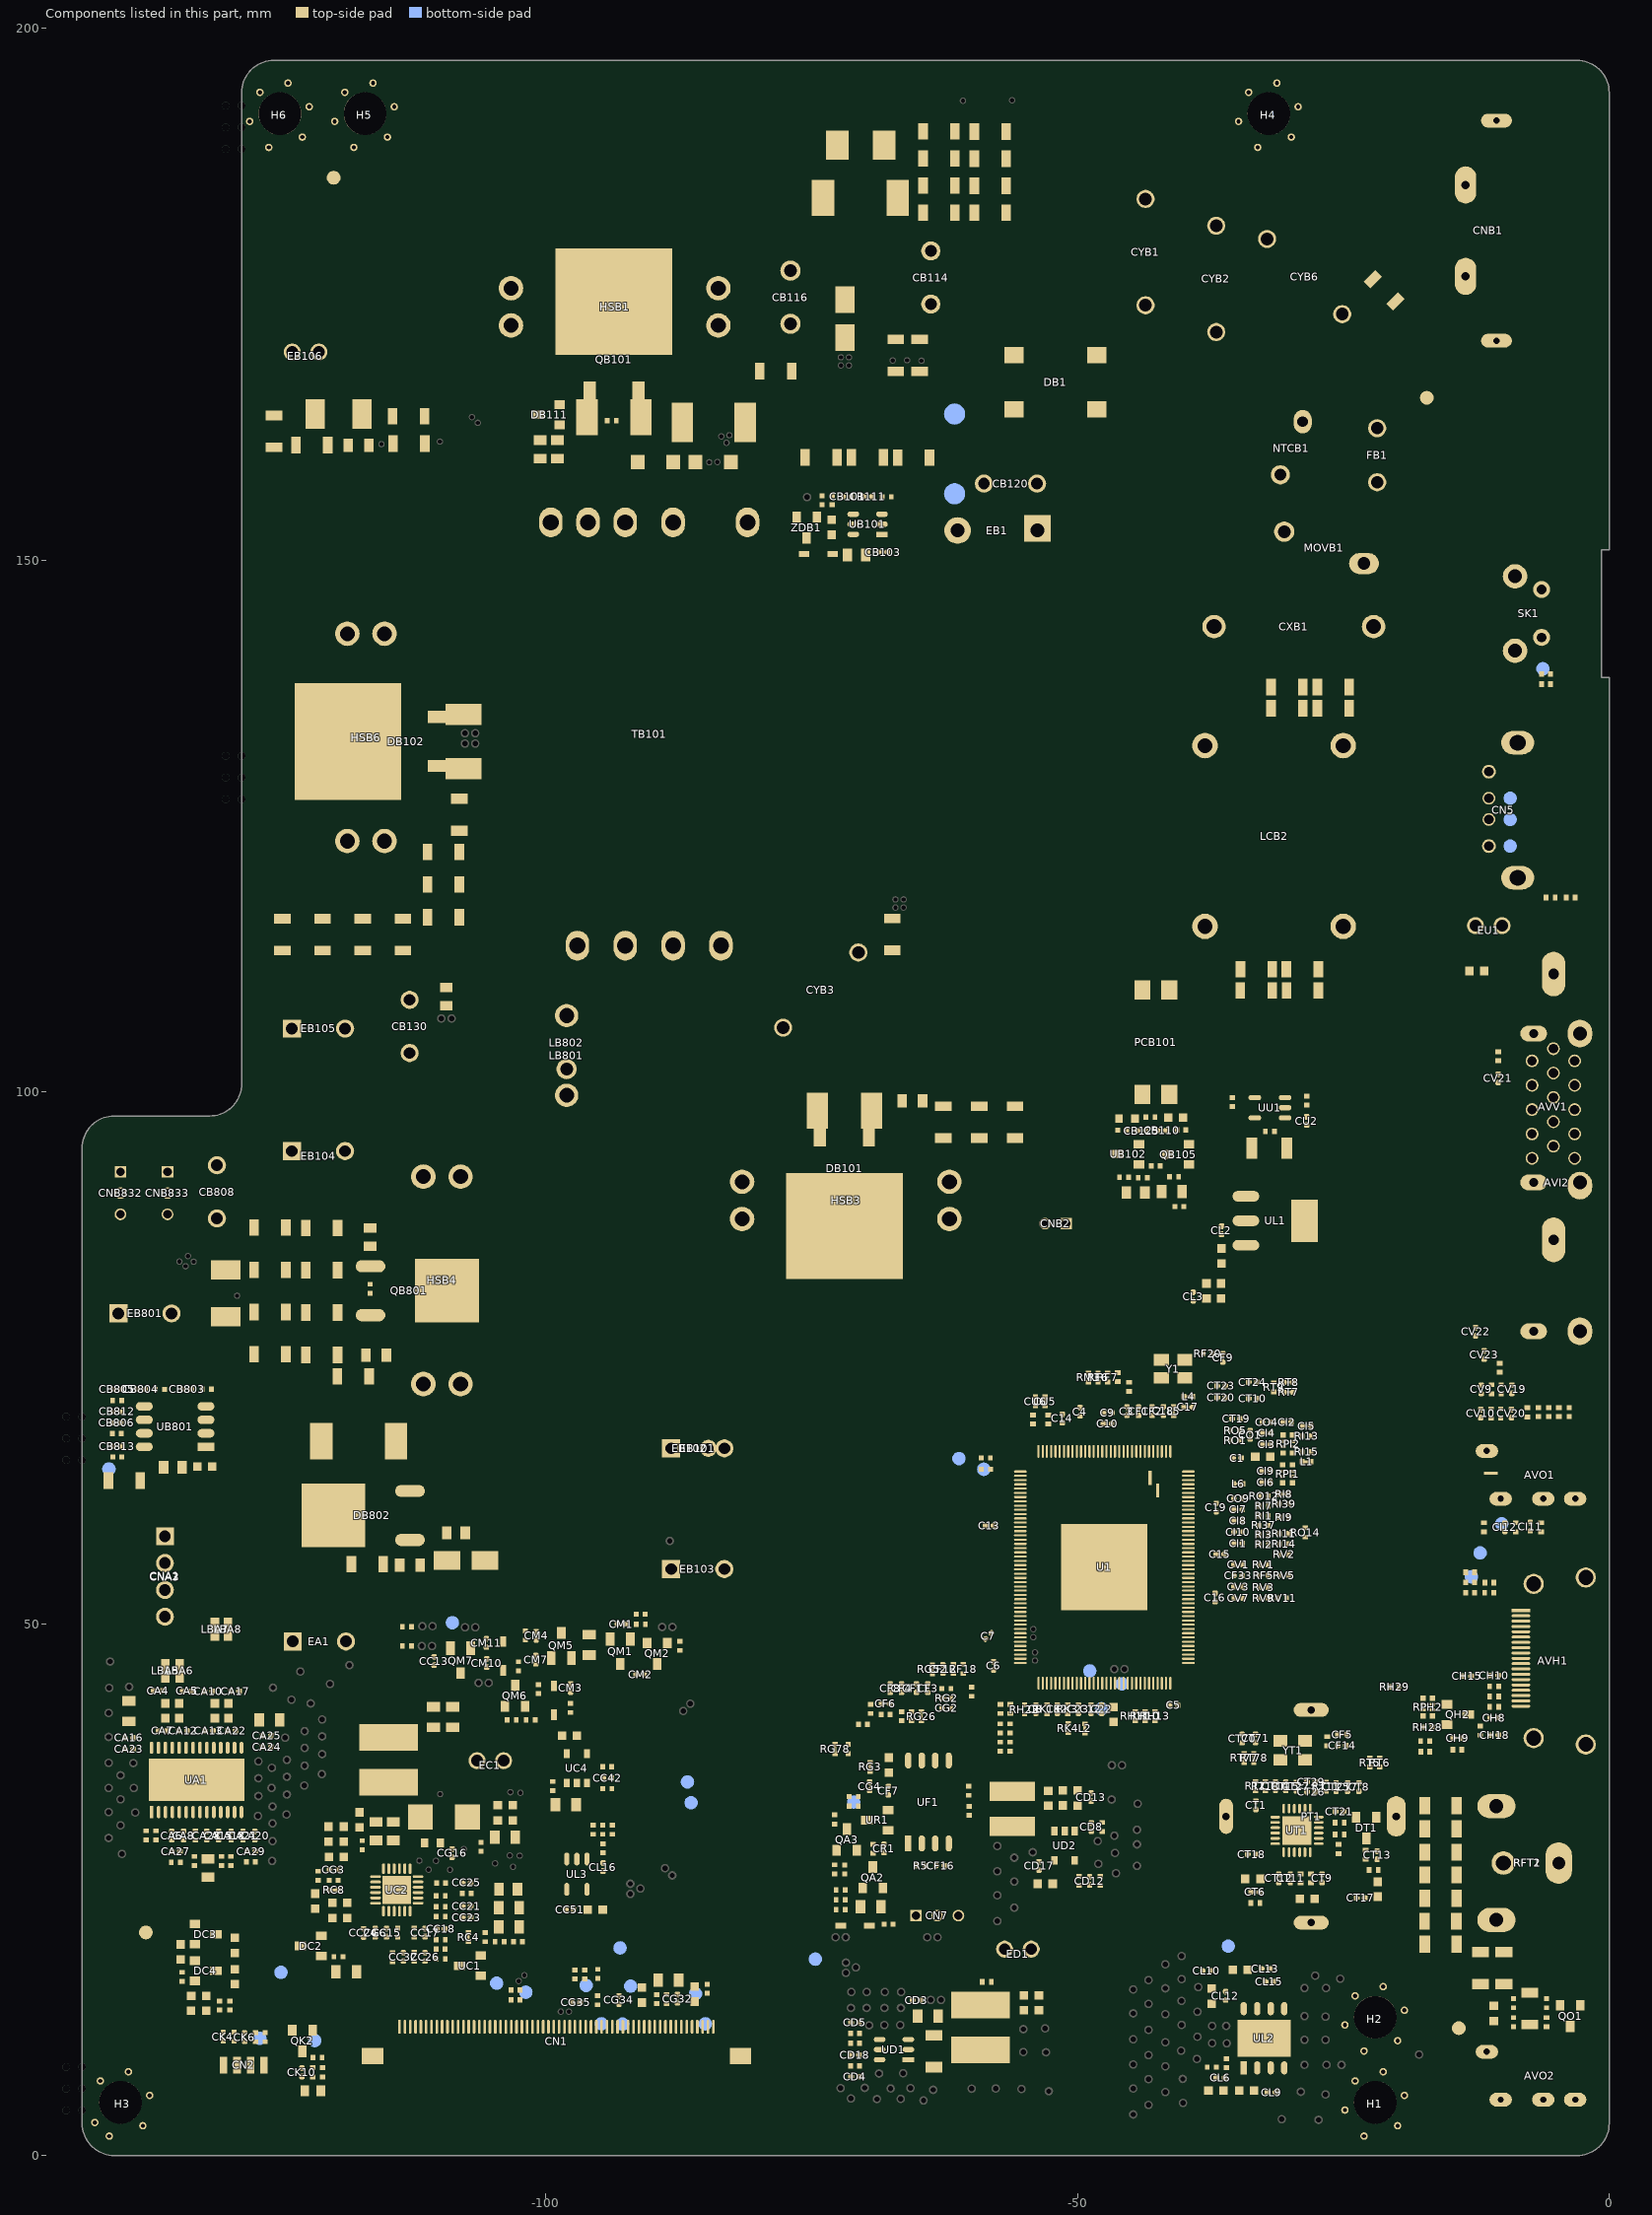
[diagram p0: the components of this part, seen from the top]
# Altium PCB MISC86383-9.PcbDoc (part 16 of 18)
Units mm, origin at the board's own origin, x right, y up, seen from the top; angles counter-clockwise.
Board outline 143.6 x 197 mm, 2 copper layers (TopLayer, BottomLayer), stack 1.571 mm thick; 743 components, 401 nets, 2996 pads, 1077 vias.
Unrouted connection lines stored in the file: 4.

## Via types
v1: diameter 0.6, hole 0.4, TopLayer to BottomLayer, tented both sides, 993 vias
v2: diameter 0.6, hole 0.4, TopLayer to BottomLayer, 65 vias
v3: diameter 0.7, hole 0.5, TopLayer to BottomLayer, tented both sides, 15 vias
v4: diameter 0.8, hole 0.5, TopLayer to BottomLayer, tented both sides, 4 vias

## Nets (pads, with @x,y where several pads share a name; then routed paths per layer and width w, separated by ;. In a path a pad name is that pad's centre, name@x,y a point inside that pad or via, vN(x,y) a via of type N, cw(c..) or ccw(c..) an arc to the next point about the centre after c; other vN are vias at no path point) (continued)
pads on no net: AI_V.0 AI_V.1 AI_V.2 AVH1.4@-2.9,39.05 AVH1.4@-2.9,53.95 AVH1.4@-7.2,39.25 AVH1.4@-7.2,53.75 AVI2.0 AVO1.0 AVO2.0 AVO2.4 AVV1.0 AVV1.4 AVV1.9 AVV1.11 AVV1.30 AVV1.31 AVV1.32 AVV1.33 AVV1.34 AVV1.35 AVV1.36 AVV1.37 AVV1.38 AVV1.39 AVV1.40 AVV1.41 AVV1.42 AVV1.43 AVV1.44 C1.2@-34.985,65.586 C3.2@-45.337,69.994 C4.2@-49.757,69.93 C5.2@-40.956,42.333 C6.2@-57.891,46.047 C7.2@-58.38,48.849 C8.2@-53.91,41.978 C9.2@-47.159,69.844 C10.2@-47.165,68.815 C12.2@-48.728,41.978 C13.2@-58.278,59.212 C14.2@-51.435,69.31 C15.2@-36.576,56.54 C16.2@-37.059,52.476 C17.2@-39.586,70.371 C18.2@-41.912,70.002 C19.2@-36.944,60.935 C22.2@-47.725,41.978 C23.2@-49.909,41.978 CA4.2@-136.495,43.698 CA5.2@-133.739,43.673 CA6.2@-135.182,30.083 CA7.2@-136.045,39.939 CA8.2@-134.064,30.083 CA10.2@-131.732,43.66 CA12.2@-134.115,39.939 CA13.2@-131.676,39.939 CA15.2@-130.762,30.083 CA16.2@-139.191,39.278 CA17.2@-129.205,43.66 CA18.2@-129.594,30.083 CA20.2@-127.358,30.083 CA21.2@-128.476,30.083 CA22.2@-129.543,39.939 CA23.2@-139.191,38.212 CA24.2@-126.233,38.427 CA25.2@-126.233,39.494 CA27.2@-134.782,28.598 CA28.2@-131.88,30.084 CA29.2@-127.71,28.604 CB101.2@-71.641,155.994 CB103.2@-68.288,150.774 CB110.2@-42.062,96.393 CB111.2@-69.736,155.994 CB114.1@-63.792,174.093 CB114.1@-63.792,179.094 CB116.0 CB120.41 CB120.42 CB125.2@-43.968,96.368 CB130.3 CB130.4 CB803.2@-133.737,72.074 CB804.2@-138.075,72.06 CB805.2@-140.31,72.047 CB806.2@-140.345,68.885 CB808.41 CB808.42 CB812.2@-140.341,69.952 CB813.2@-140.319,66.675 CC13.2@-110.503,46.495 CC15.2@-114.98,20.955 CC17.2@-111.36,20.955 CC18.2@-109.884,21.302 CC21.2@-107.443,23.463 CC23.2@-107.444,22.396 CC24.2@-117.129,20.937 CC25.2@-107.449,25.645 CC26.2@-111.36,18.669 CC32.2@-113.392,18.669 CC42.2@-94.208,35.497 CC51.2@-97.739,23.114 CD3.2@-65.125,14.605 CD4.2@-70.917,7.417 CD5.2@-70.919,12.49 CD8.2@-48.701,30.889 CD12.2@-48.854,25.82 CD13.2@-48.717,33.693 CD17.2@-53.619,27.229 CD18.2@-70.92,9.451 CF1.2@-44.249,69.977 CF2.2@-42.979,69.989 CF3.2@-64.069,43.946 CF4.2@-66.548,43.942 CF6.2@-68.047,42.469 CF7.2@-67.783,34.296 CF8.2@-67.615,43.942 CF9.2@-36.332,75.011 CF11.2@-65.151,43.942 CF12.2@-62.649,45.745 CF14.2@-25.11,38.547 CF16.2@-62.883,27.254 CF33.2@-34.891,54.524 CG2.2@-62.332,42.05 CG3.2@-119.957,26.878 CG4.2@-69.545,34.722 CG6.2@-116.046,20.955 CG16.2@-108.814,28.435 CG32.2@-87.617,14.745 CG34.2@-93.116,14.618 CG35.2@-97.168,14.402 CH8.2@-10.821,41.166 CH9.2@-14.276,39.261 CH10.2@-10.82,45.149 CH15.2@-13.373,45.072 CH18.2@-10.796,39.54 CI1.2@-34.882,57.572 CI2.2@-30.281,68.963 CI3.2@-32.203,66.874 CI4.2@-32.203,67.936 CI5.2@-28.447,68.595 CI6.2@-32.267,63.29 CI7.2@-34.882,60.734 CI8.2@-34.882,59.705 CI9.2@-32.267,64.357 CI10.2@-34.882,58.638 CI11.2@-7.417,59.131 CI12.2@-9.804,59.08 CK2.2@-51.903,41.978 CK4.2@-130.333,11.174 CK6.2@-128.321,11.125 CK10.2@-122.936,7.823 CL2.2@-36.449,86.991 CL3.2@-39.116,80.772 CL6.2@-36.55,7.315 CL9.2@-31.75,5.944 CL10.2@-37.846,17.374 CL12.2@-36.068,15.012 CL13.2@-32.309,17.577 CL15.2@-31.953,16.358 CL16.2@-94.615,27.114 CM1.2@-92.9,49.975 CM2.2@-91.122,45.212 CM3.2@-97.665,43.963 CM4.2@-100.901,48.869 CM7.2@-100.94,46.622 CM10.2@-105.55,46.304 CM11.2@-105.588,48.197 CN1.20 CN1.21 CN1.22 CN1.23 CN1.24 CN1.25 CN1.26 CN1.27 CN1.28 CN1.29 CN1.30 CN1.31 CN1.32 CN1.33 CN1.43 CN1.55 CN5.0 CN5.1@-11.31,125.63 CN5.2@-11.31,127.63 CN5.3@-11.31,130.13 CN7.0 CNA1.0 CNA2.0 CNA3.0 CNB1.0 CNB1.1@-10.6,170.65 CNB1.1@-10.6,191.35 CNB1.1@-13.5,176.7 CNB1.1@-13.5,185.3 CNB1.3 CNB1.4 CNB2.0 CNB832.0 CNB832.2 CNB833.0 CNB833.2 CO1.2@-33.752,67.769 CO4.2@-32.208,68.951 CO9.2@-34.882,61.788 CR1.2@-68.191,28.866 CT1.2@-33.225,32.933 CT6.2@-33.289,24.767 CT7.2@-24.597,34.648 CT8.2@-23.53,34.648 CT9.2@-26.997,26.062 CT10.2@-33.521,71.184 CT11.2@-29.987,26.063 CT12.2@-31.067,26.062 CT13.2@-21.831,28.24 CT14.2@-31.379,34.736 CT15.2@-30.414,34.71 CT17.2@-23.374,24.216 CT18.2@-33.614,28.323 CT19.2@-35.085,69.27 CT20.2@-36.487,71.26 CT21.2@-25.372,32.348 CT23.2@-36.487,72.371 CT24.2@-33.521,72.721 CT25.2@-25.677,34.648 CT26.2@-28.026,34.203 CT27.2@-29.436,34.698 CT29.2@-28.026,35.13 CT70.2@-34.52,39.204 CT71.2@-33.266,39.229 CU2.2@-28.448,97.286 CV1.2@-34.883,55.547 CV3.2@-34.883,53.464 CV7.2@-34.87,52.397 CV9.2@-12.032,72.056 CV10.2@-12.084,69.775 CV19.2@-9.155,72.056 CV20.2@-9.195,69.781 CV21.2@-10.439,101.289 CV22.2@-12.56,77.47 CV23.2@-11.747,75.285 CXB1.77 CXB1.78 CYB1.61 CYB2.61 CYB3.61 CYB6.61 DB802.4 EA1.0 EA1.1@-118.798,48.336 EA1.1@-123.798,48.336 EB1.1@-53.775,152.801 EB1.1@-61.275,152.801 EB101.0 EB101.1@-83.212,66.497 EB101.1@-88.212,66.497 EB102.1@-84.712,66.497 EB102.1@-88.212,66.497 EB103.0 EB103.1@-83.212,55.143 EB103.1@-88.212,55.143 EB104.0 EB104.1@-118.874,94.45 EB104.1@-123.874,94.45 EB105.0 EB105.1@-118.874,105.969 EB105.1@-123.874,105.969 EB106.0 EB801.0 EB801.1@-135.193,79.184 EB801.1@-140.193,79.184 EC1.0 EC1.5 EC1.6 ED1.0 ED1.5 ED1.6 EU1.0 EU1.5 EU1.6 FB1.4 FB1.5 GD1.0 GD2.0 GD3.0 H1.0 H2.0 H3.0 H4.0 H5.0 H6.0 HSB1.0 HSB3.0 HSB4.0 HSB6.0 LB801.1@-98.044,99.692 LB801.1@-98.044,107.191 LB802.3 LB802.4 LCB2.0 M1.0 M2.0 M3.0 M4.0 Manufacture_Info.0 MOVB1.2@-23.06,149.694 MOVB1.2@-30.56,152.694 NTCB1.2@-30.92,158.041 NTCB1.3 PCB101及周围贴片器件.0 PT1.0 RB101,102,143,144电阻附近.0 RFT1.0 RFT2.0 S/N1.0 S/N2.0 SK1.0 TB101.0 TB101.4 U1.1@-45.021,52.513 U1.1@-45.021,55.313 U1.1@-45.021,58.113 U1.1@-47.471,52.513 U1.1@-47.471,55.313 U1.1@-47.471,58.113 U1.1@-49.921,52.513 U1.1@-49.921,55.313 U1.1@-49.921,58.113 U1.31 U1.58 U1.128 U1.130 U1.131 U1.134 UA1.13 UA1.EPAD@-130.418,34.641 UA1.EPAD@-130.418,35.991 UA1.EPAD@-132.036,34.641 UA1.EPAD@-132.036,35.991 UA1.EPAD@-133.654,34.641 UA1.EPAD@-133.654,35.991 UA1.EPAD@-135.272,34.641 UA1.EPAD@-135.272,35.991 UB101及周围贴片器件.0 UB801及周围贴片器件.0 UL3.4 UT1.14 UT1.21 XCM101B1-PT.0 XXXXXX.0 XXXXXXXXXXXXXXX.0 用于U1上.0
copper on no net: | length 86.4
  TopLayer w0.127: 114.211,36.124 114.211,38.124 ; 100.218,36.124 118.812,36.124 118.812,38.124 100.218,38.124 100.218,36.124
  BottomLayer w0.127: 114.211,30.59 114.211,32.59 ; 100.218,30.59 100.218,32.59 118.812,32.59 118.812,30.59 100.218,30.59

## Polygon pours and split planes (outlines as drawn)
GND on BottomLayer "5" (solid, remove dead copper, pour order 1135): -60.452,27.432 -53.645,34.239 -50.59,34.239 -38.415,34.239 -36.938,32.762 -43.536,26.164 -43.536,23.266 -45.466,23.266 -46.126,22.606
GND on BottomLayer "5" (solid, remove dead copper, pour order 1133): -95.336,26.504 -95.336,35.438 -91.789,38.986 -91.071,39.704 -86.042,39.704 -84.561,41.185 -84.561,43.296 -84.83,43.296 -86.267,44.732 -87.472,45.938 -87.472,48.224 -87.472,49.055 -87.405,49.122 -87.334,49.193 -87.334,49.793 -87.123,50.005 -84.78,50.005 -59.301,50.005 -49.758,40.462 -49.778,40.442 -49.778,37.207 -48.681,37.207 -46.812,35.338 -44.212,32.739 -44.212,25.944 -71.798,25.944 -75.081,29.227 -76.659,30.805 -87.958,30.805 -93.577,30.805 -94.902,29.479 -95.281,29.101 -95.281,26.765
GND on BottomLayer "5" (solid, remove dead copper, pour order 1132): -44.793,35.457 -44.856,35.521 -44.856,37.96 -44.856,45.94 -45.557,46.641 -45.688,46.772 -46.216,46.772 -46.663,47.22 -46.663,47.892 -52.414,53.642 -52.414,63.301 -52.414,78.379 -50.654,80.139 -50.035,80.757 -47.039,80.757 -24.326,80.757 -16.705,73.136 -11.612,68.043 -11.612,59.599 -11.612,59.31 -9.469,57.167 -9.469,43.141 -13.565,39.045 -25.822,26.789 -40.53,26.789 -41.409,26.789 -41.732,27.112
RFGND on BottomLayer "12" (solid, remove dead copper, pour order 1124): 2.707,19.796 -11.576,19.796 cw(c-11.576,22.336) -14.116,22.336 -14.116,22.881 -14.116,33.438 cw(c-13.193,33.438) -13.193,34.361 2.071,34.361 cw(c2.071,34.329) 2.103,34.329 2.421,34.329
GND on BottomLayer "12" (solid, remove dead copper, pour order 1129): -143.6,0 -143.6,61.314 -143.446,61.468 -143.269,61.646 -140.525,61.646 -132.601,61.646 -129.311,58.356 -127,56.045 -127,55.27 -123.8,52.07 -119.99,52.07 -94.767,52.07 -92.24,54.597 -91.618,55.22 -88.25,55.22 -79.858,55.22 -79.096,54.458 -77.368,54.458 -72.657,59.169 -50.546,81.28 -33.757,81.28 -32.855,81.28 -30.264,83.871 -26.683,87.452 -26.683,100.838 -26.683,101.092 -21.895,105.88 -13.437,114.338 -13.437,118.415 -13.437,133.452 -13.437,134.595 -13.208,134.823 -11.849,136.182 -11.798,136.233 -11.798,141.008 -11.798,152.324 -9.906,154.216 -4.153,159.969 -2.121,159.969 0.457,159.969 1.156,159.271 1.448,158.979 1.448,153.06 1.448,0.648 -1.041,-1.841 -1.308,-1.575 -129.857,-1.575 -142.025,-1.575 -143.6,0
VBL on BottomLayer "12" (solid, remove dead copper, pour order 1115): -126.695,150.089 -114.059,150.089 -109.588,145.618 -105.232,141.262 -105.232,137.262 -105.232,135.953 -105.372,135.814 -105.778,135.407 -106.591,135.407 -108.128,135.407 -108.598,134.937 -108.89,134.645 -108.89,134.137 -108.89,131.064 -106.515,128.689 -104.064,126.238 -104.064,119.355 -104.064,112.077 -104.851,111.29 -105.435,110.706 -107.01,110.706 -110.731,110.706 -111.354,111.328 -111.658,111.633 -112.738,111.633 -115.799,111.633 -116.624,110.807 -120.193,107.239 -121.895,107.239 -122.352,107.239 -123.012,106.578 -123.952,105.639 -126.365,105.639 -127.432,105.639 -127.94,106.147 -128.575,106.782 -128.575,107.226 -128.575,148.361 -127.051,149.885 -126.848,150.089 -126.695,150.089
D_QB801 on BottomLayer "12" (solid, remove dead copper, pour order 1119): -105.143,106.591 -102.07,106.591 -100.635,106.591 -99.593,105.55 -98.92,104.877 -97.701,104.877 -95.275,104.877 -94.132,103.734 -94.132,102.21 -94.132,60.541 -95.466,59.207 -96.863,57.81 -101.74,57.81 -105.842,57.81 -108.306,60.274 -110.274,62.243 -110.274,65.697 -110.274,67.92 -112.344,69.99 -113.982,71.628 -113.982,79.743 -113.982,88.049 -114.567,88.633 -115.037,89.103 -115.037,90.284 -115.037,97.638 -111.442,101.232 -106.083,106.591 -105.143,106.591
12V on BottomLayer "12" (solid, remove dead copper, pour order 1120): -87.262,100.292 -69.748,100.292 -65.583,96.126 -53.988,96.126 -52.375,94.513 -52.375,84.785 -71.653,65.507 -76.797,65.507 -89.154,77.864 -89.154,98.4
D_QB101 on BottomLayer "12" (solid, remove dead copper, pour order 1117): -95.809,197 -72.883,197 -71.806,195.923 -71.666,195.783 -71.666,195.148 -71.666,186.576 -71.069,185.979 -70.218,185.128 -70.218,184.15 -70.218,181.28 -69.342,180.403 -67.259,178.321 -67.259,177.368 -67.259,176.276 -67.589,175.946 -67.932,175.603 -68.605,175.603 -79.019,175.603 -80.404,174.219 -81.432,173.19 -81.432,171.679 -81.432,169.456 -82.105,168.783 -82.232,168.656 -85.077,168.656 -86.525,168.656 -87.376,167.805 -90.462,164.719 -94.196,164.719 -102.946,164.719 -104.419,166.192 -105.575,167.348 -106.566,167.348 -114.008,167.348 -116.307,169.647 -116.764,170.104 -116.764,172.136 -116.764,174.041 -116.421,174.384 -116.129,174.676 -115.621,174.676 -109.868,174.676 -104.991,179.553 -99.746,184.798 -99.746,188.671 -99.746,194.475 -98.171,196.05 -97.221,197 -95.771,197
SGND on BottomLayer "12" (solid, remove dead copper, pour order 1114): -73.685,156.642 -66.84,156.642 -66.357,156.159 -66.142,155.943 -66.142,155.359 -66.142,152.87 -67.081,151.93 -68.694,150.317 -69.85,150.317 -74.612,150.317 -75.755,151.46 -76.441,152.146 -76.441,152.246 -76.441,152.438 -75.717,153.162 -75.717,156.108 -75.514,156.312 -75.184,156.642 -73.685,156.642
GND on BottomLayer "12" (solid, remove dead copper, pour order 1116): -135.585,74.549 -130.2,69.164 -130.2,64.325 -130.492,64.033 -137.058,64.033 -138.392,62.7 -143.027,62.7 -143.675,63.348 -143.675,70.955 -140.081,74.549
GND on BottomLayer "12" (solid, remove dead copper, pour order 1113): -26.683,101.092 -47.737,80.038 -47.737,76.33 -46.876,77.191 -22.86,77.191 -22.86,89.865 -21.514,91.211 -23.317,93.015 -23.317,97.155 -23.317,98.044 -24.536,99.263
GND on BottomLayer "12" (solid, remove dead copper, pour order 1112): -38.303,87.478 -38.303,98.984 -37.313,99.974 -36.982,100.305 -29.972,100.305 -22.758,100.305 -22.403,99.949 -29.616,92.735 -29.616,90.322 -29.667,90.272
GND on TopLayer "7" (solid, remove dead copper, pour order 1134): -34.068,51.897 -34.068,55.941 -33.882,56.128 -32.521,56.128 -31.426,57.222 -31.041,57.607 -30.189,57.607 -26.132,57.607 -22.878,60.862 -21.65,62.089 -20.224,62.089 -19.264,62.089 -18.551,62.802 -18.551,70.766 -14.589,74.728 -14.157,75.16 -14.157,78.12 -14.157,78.742 -11.346,81.553 -11.346,82.021 -11.346,101.743 -8.93,104.159 -8.177,104.912 -7.839,104.912 -7.839,94.626 -8.505,93.96 -8.505,76.759 -13.71,71.554 -15.639,69.625 -15.639,67.213 -15.639,61.165 -17.642,59.163 -17.668,59.136 -20.863,59.136 -26.551,53.448 -28.336,53.448 -29.851,51.934 -31.638,51.934 -33.952,51.934 -33.973,51.913
GND on TopLayer "5" (solid, remove dead copper, pour order 1131): -38.539,45.924 -38.539,50.313 -38.01,50.842 -37.473,51.379 -36.373,51.379 -9.732,51.379 -9.663,51.311 -9.414,51.062 -9.414,46.356 -9.414,45.455 -9.651,45.218 -10.325,45.218 -10.482,45.376 -11.151,46.045 -11.524,46.045 -38.361,46.045 -38.497,45.909
GND on TopLayer "5" (solid, remove dead copper, pour order 1130): -114.173,10.909 -113.928,11.154 -113.25,11.154 -104.436,11.154 -104.418,11.173 -84.827,11.173 -83.756,12.243 -83.185,12.814 -83.185,14.618 -83.185,42.939 -79.87,46.253 -62.293,63.83 -61.658,63.83 -57.379,63.83 -56.655,63.106 -56.274,62.726 -56.274,62.265 -56.274,55.131 -56.223,55.08 -57.785,55.08 -58.102,54.762 -73.825,39.04 -73.825,32.69 -73.825,6.337 -74.917,5.245 -76.157,4.005 -76.722,4.005 -110.926,4.005 -112.751,5.829 -114.338,7.417 -114.338,9.779 -114.338,10.706 -114.071,10.973
GND on TopLayer "5" (solid, remove dead copper, pour order 1127): -7.281,123.557 -7.281,125.713 -7.163,125.832 -5.639,125.832 -4.623,124.816 -3.81,124.003 -3.81,122.936 -3.81,119.635 -3.199,119.025 -3.199,117.141 -7.8,112.54 -7.8,110.338 -7.8,108.071 -9.398,106.473 -11.836,104.034 -11.836,95.809 -11.836,81.737 -14.783,78.791 -16.053,77.521 -17.374,77.521 -18.278,78.425 -31.445,78.425 -43.129,78.425 -46.116,75.438 -46.391,75.163 -49.29,75.163 -51.918,72.535 -51.918,70.866 -51.918,70.104 -51.664,69.85 -51.714,69.799 -51.714,68.682 -52.222,68.174 -53.899,68.174 -53.932,68.174 -54.601,68.843 -54.458,68.986 -54.458,71.628 -54.458,72.085 -53.645,72.898 -49.886,76.657 -49.124,76.657 -47.049,76.657 -46.685,77.021 -44.378,79.328 -44.153,79.553 -39.421,79.553 -25.146,79.553 -24.689,80.01 -16.053,80.01 -13.411,82.652 -13.411,84.328 -13.462,84.379 -13.312,84.529 -13.312,104.394 -9.373,108.333 -9.373,108.56 -9.373,114.072 -5.994,117.451 -5.994,119.228 -5.994,122.682 -6.706,123.393
GND on TopLayer "5" (solid, remove dead copper, pour order 1126): -51.32,46.547 -52.071,46.547 -52.884,47.36 -52.884,57.938 -52.634,58.188 -52.634,62.918 -52.276,63.276 -49.188,63.276 -48.962,63.05 -48.857,62.945 -47.981,62.945 -47.954,62.945 -47.204,63.695 -46.284,64.615 -45.165,64.615 -42.238,64.615 -41.329,64.615 -40.847,64.132 -40.644,63.929 -40.644,62.603 -40.644,47.353 -41.331,46.665 -41.864,46.132 -43.611,46.132 -44.87,46.132 -45.551,46.813 -45.684,46.68 -50.925,46.68
RFGND on TopLayer "12" (solid, remove dead copper, pour order 1125): 2.275,17.582 -13.368,17.582 cw(c-13.368,19.892) -15.678,19.892 -15.678,33.201 cw(c-14.249,33.201) -14.249,34.631 0.608,34.631 0.878,34.631 cw(c0.878,32.091) 3.418,32.091 3.418,22.321 3.418,18.716 cw(c2.265,18.716) 2.265,17.563
GND on TopLayer "12" (solid, remove dead copper, pour order 1128): -143.6,0 -143.6,61.314 -143.446,61.468 -143.269,61.646 -140.525,61.646 -132.601,61.646 -129.311,58.356 -127,56.045 -127,55.27 -123.8,52.07 -119.99,52.07 -94.767,52.07 -92.24,54.597 -91.618,55.22 -88.25,55.22 -79.858,55.22 -79.096,54.458 -77.368,54.458 -72.657,59.169 -50.546,81.28 -33.757,81.28 -32.855,81.28 -30.264,83.871 -26.683,87.452 -26.683,100.838 -26.683,101.092 -21.895,105.88 -13.437,114.338 -13.437,118.415 -13.437,133.452 -13.437,134.595 -13.208,134.823 -11.849,136.182 -11.798,136.233 -11.798,141.008 -11.798,152.324 -9.906,154.216 -4.153,159.969 -2.121,159.969 0.457,159.969 1.156,159.271 1.448,158.979 1.448,153.06 1.448,0.648 -1.041,-1.841 -1.308,-1.575 -129.857,-1.575 -142.025,-1.575 -143.6,0
D_QB101 on TopLayer "12" (solid, remove dead copper, pour order 1118): -101.321,197 -72.261,197 -71.615,196.355 -71.463,196.202 -71.463,195.707 -71.463,186.449 -70.396,185.382 -70.244,185.229 -70.244,184.556 -70.244,180.911 -69.088,179.756 -67.475,178.143 -67.475,176.187 -67.475,175.831 -67.983,175.323 -70.129,173.177 -71.133,173.177 -73.05,173.177 -73.596,173.723 -75.489,175.616 -76.505,175.616 -78.765,175.616 -79.553,174.828 -80.543,173.838 -80.543,173.406 -80.543,172.225 -81.102,171.666 -83.591,169.177 -88.303,169.177 -98.844,169.177 -99.949,168.072 -100.863,167.157 -103.708,167.157 -111.811,167.157 -113.805,169.151 -116.027,171.374 -116.027,178.054 -116.027,179.578 -114.998,180.607 -114.871,180.734 -114.046,180.734 -111.963,180.734 -109.118,183.578 -105.778,186.919 -105.778,189.598 -105.778,194.945 -104.775,195.948 -103.723,197 -101.536,197
VBL on TopLayer "12" (solid, remove dead copper, pour order 1121): -125.603,150.139 -125.59,150.127 -114.008,150.127 -111.912,148.031 -107.251,143.37 -107.251,141.351 -107.251,137.782 -107.366,137.668 -107.404,137.63 -108.09,137.63 -111.887,137.63 -111.989,137.528 -112.116,137.401 -112.116,137.058 -112.116,129.578 -110.782,128.245 -110.16,127.622 -110.16,125.019 -110.16,115.71 -110.49,115.379 -110.82,115.049 -111.658,115.049 -127.521,115.049 -128.6,116.129 -128.6,117.119 -128.6,148.539 -127.33,149.809 -127,150.139 -125.603,150.139
12V on TopLayer "12" (solid, remove dead copper, pour order 1122): -87.338,101.067 -87.312,101.092 -82.245,101.092 -79.553,98.4 -75.247,94.094 -72.25,94.094 -68.428,94.094 -67.259,95.263 -66.04,96.482 -63.208,96.482 -53.073,96.482 -52.629,96.037 -52.387,95.796 -52.387,95.504 -52.387,82.169 -52.387,82.017 -65.532,68.872 -75.247,59.157 -77.762,59.157 -78.753,59.157 -79.4,59.804 -79.819,60.223 -79.819,66.129 -79.819,69.151 -81.724,71.056 -82.728,72.06 -82.791,72.123 -91.91,72.123 -92.316,72.123 -92.71,72.517 -93.027,72.834 -93.027,73.152 -93.027,97.815 -91.938,98.905 -89.776,101.067 -87.338,101.067
D_QB801 on TopLayer "12" (solid, remove dead copper, pour order 1123): -105.181,106.782 -100.279,106.782 -99.289,105.791 -98.501,105.004 -95.961,105.004 -95.186,105.004 -94.551,104.369 -93.713,103.53 -93.713,102.679 -93.713,71.933 -92.481,70.701 -91.402,69.621 -91.402,65.684 -91.402,60.389 -93.167,58.623 -96.914,54.877 -104.673,54.877 -106.921,54.877 -107.124,55.08 -107.163,55.118 -107.163,56.083 -107.163,56.959 -107.645,57.442 -108.102,57.899 -108.102,58.522 -108.102,59.614 -108.737,60.249 -110.528,62.039 -110.528,63.665 -110.528,67.97 -111.138,68.58 -112.382,69.825 -113.335,69.825 -113.83,69.825 -114.706,70.701 -115.367,71.361 -115.367,74.714 -115.367,76.543 -114.91,77 -114.084,77.826 -114.084,79.515 -114.084,87.96 -114.973,88.849 -115.151,89.027 -115.151,92.608 -115.151,96.825 -113.513,98.463 -105.194,106.782 -105.181,106.782

## Keep-outs
KeepOutLayer:
  circle w0.127: c-273.7,58 r0.003
  circle w0.127: c-273,58 r0.003
  circle w0.127: c-0.7,139 r0.003
  circle w0.127: c0,139 r0.003
  rectangle: 100.218,20.953 103.525,22.953
  lines w0.127: -145.1,9.58 ccw(c-144.35,10.33) -143.6,9.58 ; -145.1,64.135 cw(c-144.35,63.385) -143.6,64.135 ; -145.1,70.715 ccw(c-144.35,71.465) -143.6,70.715 ; -130.1,126.285 cw(c-129.35,125.535) -128.6,126.285 ; -130.1,132.865 ccw(c-129.35,133.615) -128.6,132.865 ; -130.1,187.42 cw(c-129.35,186.67) -128.6,187.42 ; 114.211,20.953 114.211,22.953 ; -145.1,3 cw(c-144.35,2.25) -143.6,3 ; -145.1,3 cw(c-148.1,3) -148.1,0 -270.7,0 cw(c-270.7,3) -273.7,3 -273.7,46 -273,46 -273,58 -273.7,58 -273.7,194 cw(c-270.7,194) -270.7,197 -133.1,197 cw(c-133.1,194) -130.1,194 ; -145.1,3 -145.1,96.25 cw(c-142.1,96.25) -142.1,99.25 -133.1,99.25 ccw(c-133.1,102.25) -130.1,102.25 -130.1,194 ; -143.6,3 ccw(c-140.6,3) -140.6,0 -3,0 ccw(c-3,3) 0,3 0,139 -0.7,139 -0.7,151 0,151 0,194 ccw(c-3,194) -3,197 -125.6,197 ccw(c-125.6,194) -128.6,194 ; -143.6,3 -143.6,94.75 cw(c-140.6,94.75) -140.6,97.75 -131.6,97.75 ccw(c-131.6,100.75) -128.6,100.75 -128.6,194 ; -130.1,194 ccw(c-129.35,194.75) -128.6,194 ; 100.218,20.953 100.218,22.953 118.812,22.953 118.812,20.953 100.218,20.953
  text "KeepOutLayer" at 104.099,21.485 h1.52
  text ".GKO" at 114.813,21.411 h1.52

## Other copper
TopLayer:
  drawing of 223 lines, arcs and shapes, not listed
  text "TopLayer" at 104.436,36.691 h1.52
  text ".GTL" at 114.837,36.582 h1.52